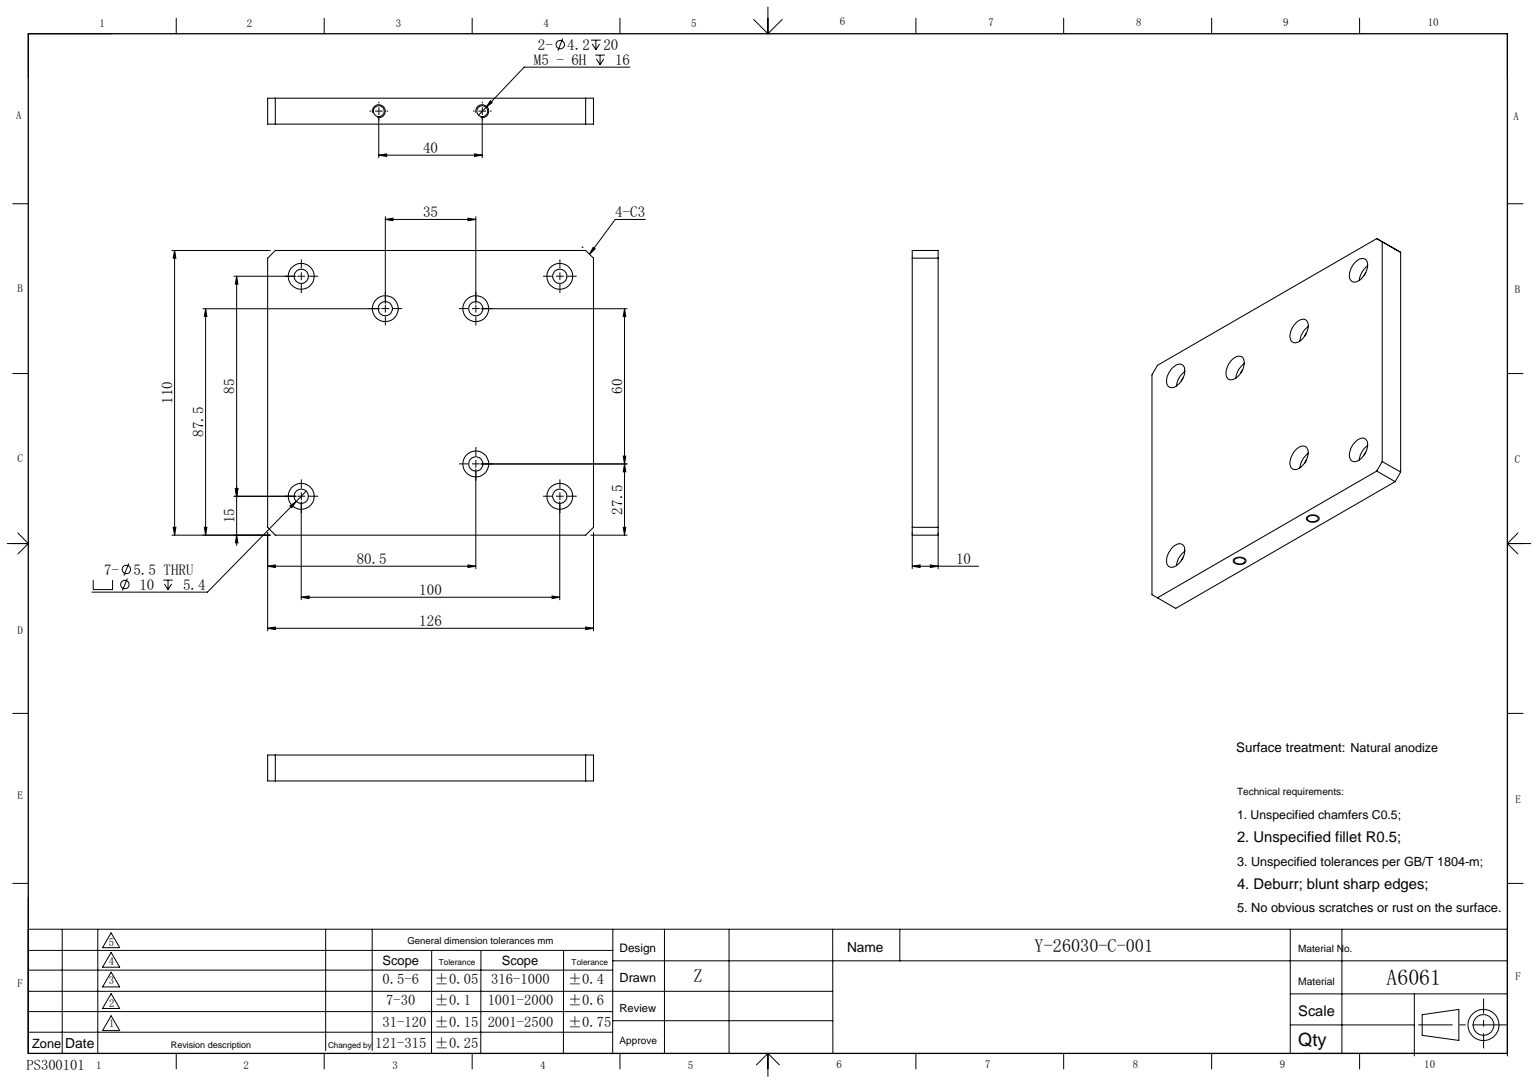
SolidWorks part; units mm, degrees
ref_plane "前视基准面" through (0, 0, 0) normal (0, 0, 1) x (1, 0, 0)
ref_plane "上视基准面" through (0, 0, 0) normal (0, 1, 0) x (1, 0, 0)
ref_plane "右视基准面" through (0, 0, 0) normal (1, 0, 0) x (0, 0, -1)
sketch "草图1" plane through (0, 0, 0) normal (0, 0, 1) x (1, 0, 0)
  line L1 (63, -55) -> (-63, -55)
  line L2 (63, -55) -> (63, 55)
  line L3 (63, 55) -> (-63, 55)
  line L4 (-63, -55) -> (-63, 55)
  line L5 (63, -55) -> (-63, 55) construction
  line L6 (63, 55) -> (-63, -55) construction
  point P0 (0, 0)
  dimension "D1" = 126
  dimension "D2" = 110
extrude "凸台-拉伸1" add sketch "草图1" along normal mid plane 10
chamfer "倒角1" distance 3 angle 45 4 edges at (-63, 55, 0) (63, 55, 0) (63, -55, 0) (-63, -55, 0)
hole_wizard "M5 六角凹头螺钉的柱形沉头孔1" positions "草图3" profile "草图2" counterbore size "M5" standard "ISO" end condition up to next
sketch "草图3" plane through (0, 0, 5) normal (0, 0, 1) x (1, 0, 0)
  point P0 (-50, 45)
  point P1 (-17.5, 32.5)
  point P2 (17.5, 32.5)
  point P3 (50, 45)
  point P4 (50, -40)
  point P5 (17.5, -27.5)
  point P6 (-50, -40)
  dimension "D1" = 50
  dimension "D2" = 17.5
  dimension "D3" = 50
  dimension "D4" = 17.5
  dimension "D5" = 45
  dimension "D6" = 32.5
  dimension "D7" = 40
  dimension "D8" = 27.5
sketch "草图2" plane through (-50, 45, 5) normal (1, 0, 0) x (0, -1, 0)
  line L0 (0, 0) -> (0, 10)
  line L1 (0, 10) -> (2.75, 10)
  line L3 (2.75, 10) -> (2.75, 5.4)
  line L4 (2.75, 5.4) -> (5, 5.4)
  line L5 (5, 5.4) -> (5, 0)
  line L7 (5, 0) -> (0, 0)
  line L11 (0, -6.35) -> (0, 107.95) construction
  dimension "通孔孔直径" = 5.5
  dimension "通孔孔深度" = 10
  dimension "柱形沉头孔直径" = 10
  dimension "柱形沉头孔深度" = 5.4
sketch "草图6" plane through (0, -55, 0) normal (0, -1, 0) x (-1, 0, 0)
  line L0 (-20, 0) -> (0, 0) construction
  line L1 (0, 0) -> (20, 0) construction
  point P0 (20, 0)
  point P2 (-20, 0)
  dimension "D1" = 20
hole_wizard "M5 螺纹孔1" positions "草图6" profile "草图7" tap size "M5" standard "ISO"
sketch "草图7" plane through (-20, -55, 0) normal (1, 0, 0) x (0, 0, -1)
  line L0 (0, 0) -> (0, 21.2618)
  line L1 (0, 21.2618) -> (2.1, 20)
  line L2 (2.1, 20) -> (2.1, 0)
  line L5 (2.1, 0) -> (0, 0)
  line L10 (0, 21.2618) -> (-2.1, 20) construction
  line L11 (0, -6.35) -> (0, 107.95) construction
  dimension "螺纹孔钻头直径" = 4.2
  dimension "螺纹孔钻头深度" = 20
  dimension "导头角度" = 118
cosmetic thread "孔螺纹线1"
cosmetic thread "孔螺纹线2"
